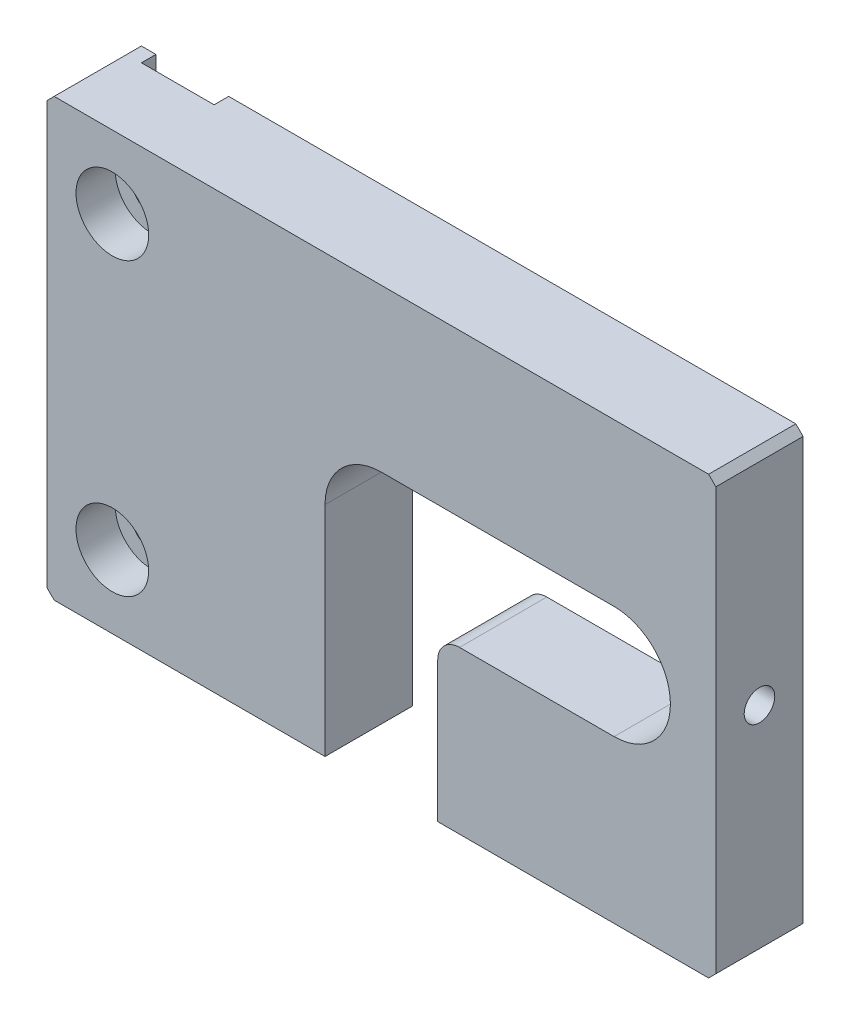
from build123d import *

# Parameters (mm, degrees)
SKETCH_1_W                     = 92
SKETCH_1_H                     = 60
EXTRUDE_1_DEPTH                = 6
CHAMFER_1_SIZE                 = 1
SKETCH_2_W                     = 10
SKETCH_2_H                     = 2
CUT_EXTRUDE_1_DEPTH            = 76.841940903
CUT_EXTRUDE_3_REACH            = 58.214
FILLET_1_R                     = 3
HOLE_WIZARD_M5_1_REACH         = 98.954
HOLE_WIZARD_M5_1_BORE_R        = 2.1
HOLE_WIZARD_M5_1_2_D           = 5.5
HOLE_WIZARD_M5_1_2_CBORE_D     = 10
HOLE_WIZARD_M5_1_2_CBORE_DEPTH = 5.4


with BuildPart() as part:
    # 草图1 → 凸台-拉伸1 (new, symmetric)
    with BuildSketch(Plane.XY):
        Rectangle(SKETCH_1_W, SKETCH_1_H)
    extrude(amount=EXTRUDE_1_DEPTH, both=True)

    # 倒角1
    chamfer_1_edges = [part.edges().sort_by_distance(p)[0] for p in [
        (-46, 30, 0),
        (46, 30, 0),
        (46, -30, 0),
        (-46, -30, 0),
    ]]
    chamfer(chamfer_1_edges, length=CHAMFER_1_SIZE)

    # 草图2 → 切除-拉伸1 (cut, through all)
    with BuildSketch(Plane(origin=(0, 30, 0), x_dir=(1, 0, 0), z_dir=(0, 1, 0))):
        with Locations((-38, 5)):
            Rectangle(SKETCH_2_W, SKETCH_2_H)
    extrude(amount=-CUT_EXTRUDE_1_DEPTH, mode=Mode.SUBTRACT)

    # 草图3 → 切除-拉伸3 (cut, up to next)
    with BuildSketch(Plane.XY.offset(6), mode=Mode.PRIVATE) as cut_extrude_3_sk1:
        with BuildLine():
            Line((7.75, 0), (7.75, -35))
            ThreePointArc((7.75, -35), (0, -42.75), (-7.75, -35))
            Line((-7.75, -35), (-7.75, 0))
            ThreePointArc((-7.75, 0), (0, 7.75), (7.75, 0))
        make_face()
    cut_extrude_3_tool1 = extrude(cut_extrude_3_sk1.sketch, amount=-CUT_EXTRUDE_3_REACH, mode=Mode.PRIVATE) & part.part
    # 草图3 → 切除-拉伸3 (cut, up to next)
    with BuildSketch(Plane.XY.offset(6), mode=Mode.PRIVATE) as cut_extrude_3_sk2:
        with BuildLine():
            Line((0, 7.75), (32, 7.75))
            ThreePointArc((32, 7.75), (39.75, 0), (32, -7.75))
            Line((32, -7.75), (0, -7.75))
            ThreePointArc((0, -7.75), (-7.75, 0), (0, 7.75))
        make_face()
    cut_extrude_3_tool2 = extrude(cut_extrude_3_sk2.sketch, amount=-CUT_EXTRUDE_3_REACH, mode=Mode.PRIVATE) & part.part
    add(cut_extrude_3_tool1.solids().sort_by_distance((0, -17.5, 6))[0], mode=Mode.SUBTRACT)
    add(cut_extrude_3_tool2.solids().sort_by_distance((16, 0, 6))[0], mode=Mode.SUBTRACT)

    # 圆角1
    fillet_1_edges = [part.edges().sort_by_distance(p)[0] for p in [
        (7.75, -7.75, 0),
    ]]
    fillet(fillet_1_edges, radius=FILLET_1_R)

    # Hole Wizard M5 _1 bore → Hole Wizard M5 _1 (cut, up to next)
    with BuildSketch(Plane(origin=(46, 0, 0), x_dir=(0, 0, -1), z_dir=(1, 0, 0)), mode=Mode.PRIVATE) as hole_wizard_m5_1_sk1:
        Circle(HOLE_WIZARD_M5_1_BORE_R)
    hole_wizard_m5_1_tool1 = extrude(hole_wizard_m5_1_sk1.sketch, amount=-HOLE_WIZARD_M5_1_REACH, mode=Mode.PRIVATE) & part.part
    add(hole_wizard_m5_1_tool1.solids().sort_by_distance((46, 0, 0))[0], mode=Mode.SUBTRACT)

    # Hole Wizard M5 _1 2 (through all)
    with Locations(Plane.XY.offset(6)):
        with Locations((-37, -20), (-37, 20)):
            CounterBoreHole(HOLE_WIZARD_M5_1_2_D / 2, HOLE_WIZARD_M5_1_2_CBORE_D / 2, HOLE_WIZARD_M5_1_2_CBORE_DEPTH)


solid = part.part
